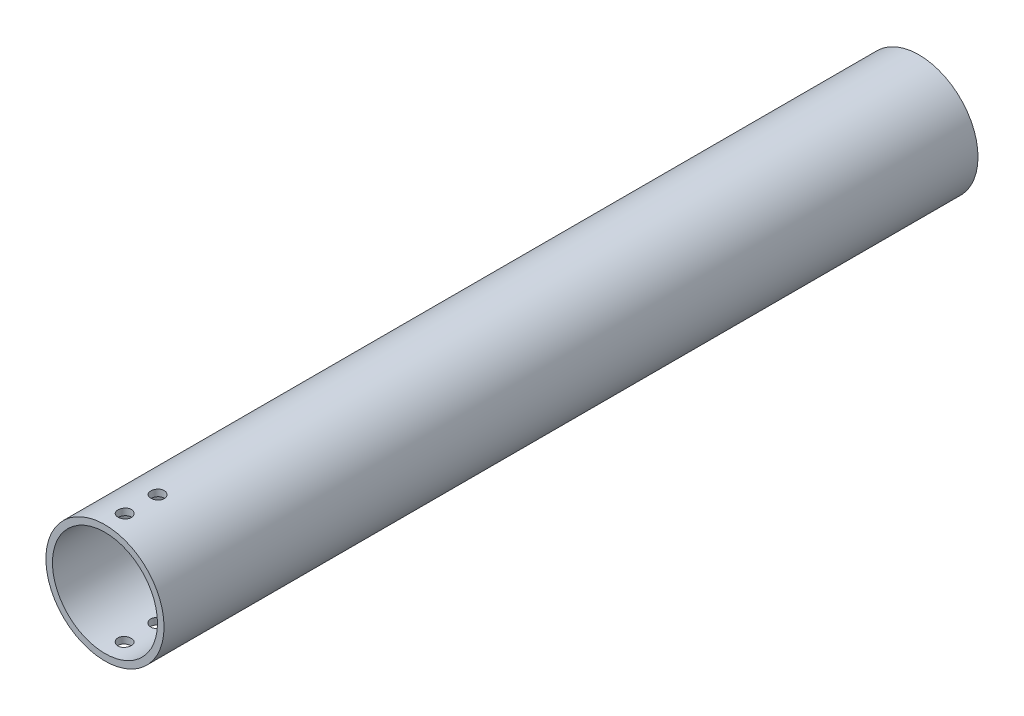
from build123d import *

# Parameters (mm, degrees)
SKETCH_1_R          = 45
SKETCH_1_R_2        = 40
EXTRUDE_1_DEPTH     = 40
SKETCH_2_R          = 50
SKETCH_2_R_2        = 40
EXTRUDE_2_DEPTH     = 30
SKETCH_3_R          = 45
SKETCH_3_R_2        = 40
EXTRUDE_3_DEPTH     = 550
SKETCH_4_R          = 5.1
CUT_EXTRUDE_1_DEPTH = 91
SKETCH_5_R          = 50
SKETCH_5_R_2        = 45
CUT_EXTRUDE_2_DEPTH = 117


with BuildPart() as part:
    # 草图1 → 凸台-拉伸1 (new body)
    with BuildSketch(Plane.XY):
        Circle(SKETCH_1_R)
        Circle(SKETCH_1_R_2, mode=Mode.SUBTRACT)
    extrude(amount=EXTRUDE_1_DEPTH)

    # 草图2 → 凸台-拉伸2 (add)
    with BuildSketch(Plane.XY.offset(40)):
        Circle(SKETCH_2_R)
        Circle(SKETCH_2_R_2, mode=Mode.SUBTRACT)
    extrude(amount=EXTRUDE_2_DEPTH)

    # 草图3 → 凸台-拉伸3 (add)
    with BuildSketch(Plane.XY.offset(70)):
        Circle(SKETCH_3_R)
        Circle(SKETCH_3_R_2, mode=Mode.SUBTRACT)
    extrude(amount=EXTRUDE_3_DEPTH)

    # 草图4 → 切除-拉伸1 (cut, symmetric)
    with BuildSketch(Plane(origin=(0, 0, 0), x_dir=(1, 0, 0), z_dir=(0, 1, 0))):
        with Locations(Location((0, -605, 0), (0, 0, 270))):
            Circle(SKETCH_4_R)
        with Locations(Location((0, -580, 0), (0, 0, 270))):
            Circle(SKETCH_4_R)
    extrude(amount=CUT_EXTRUDE_1_DEPTH, both=True, mode=Mode.SUBTRACT)

    # 草图5 → 切除-拉伸2 (cut)
    with BuildSketch(Plane(origin=(0, 0, 40), x_dir=(-1, 0, 0), z_dir=(0, 0, -1))):
        Circle(SKETCH_5_R)
        with Locations(Location((0, 0, 0), (0, 0, 180))):
            Circle(SKETCH_5_R_2, mode=Mode.SUBTRACT)
    extrude(amount=-CUT_EXTRUDE_2_DEPTH, mode=Mode.SUBTRACT)


solid = part.part
